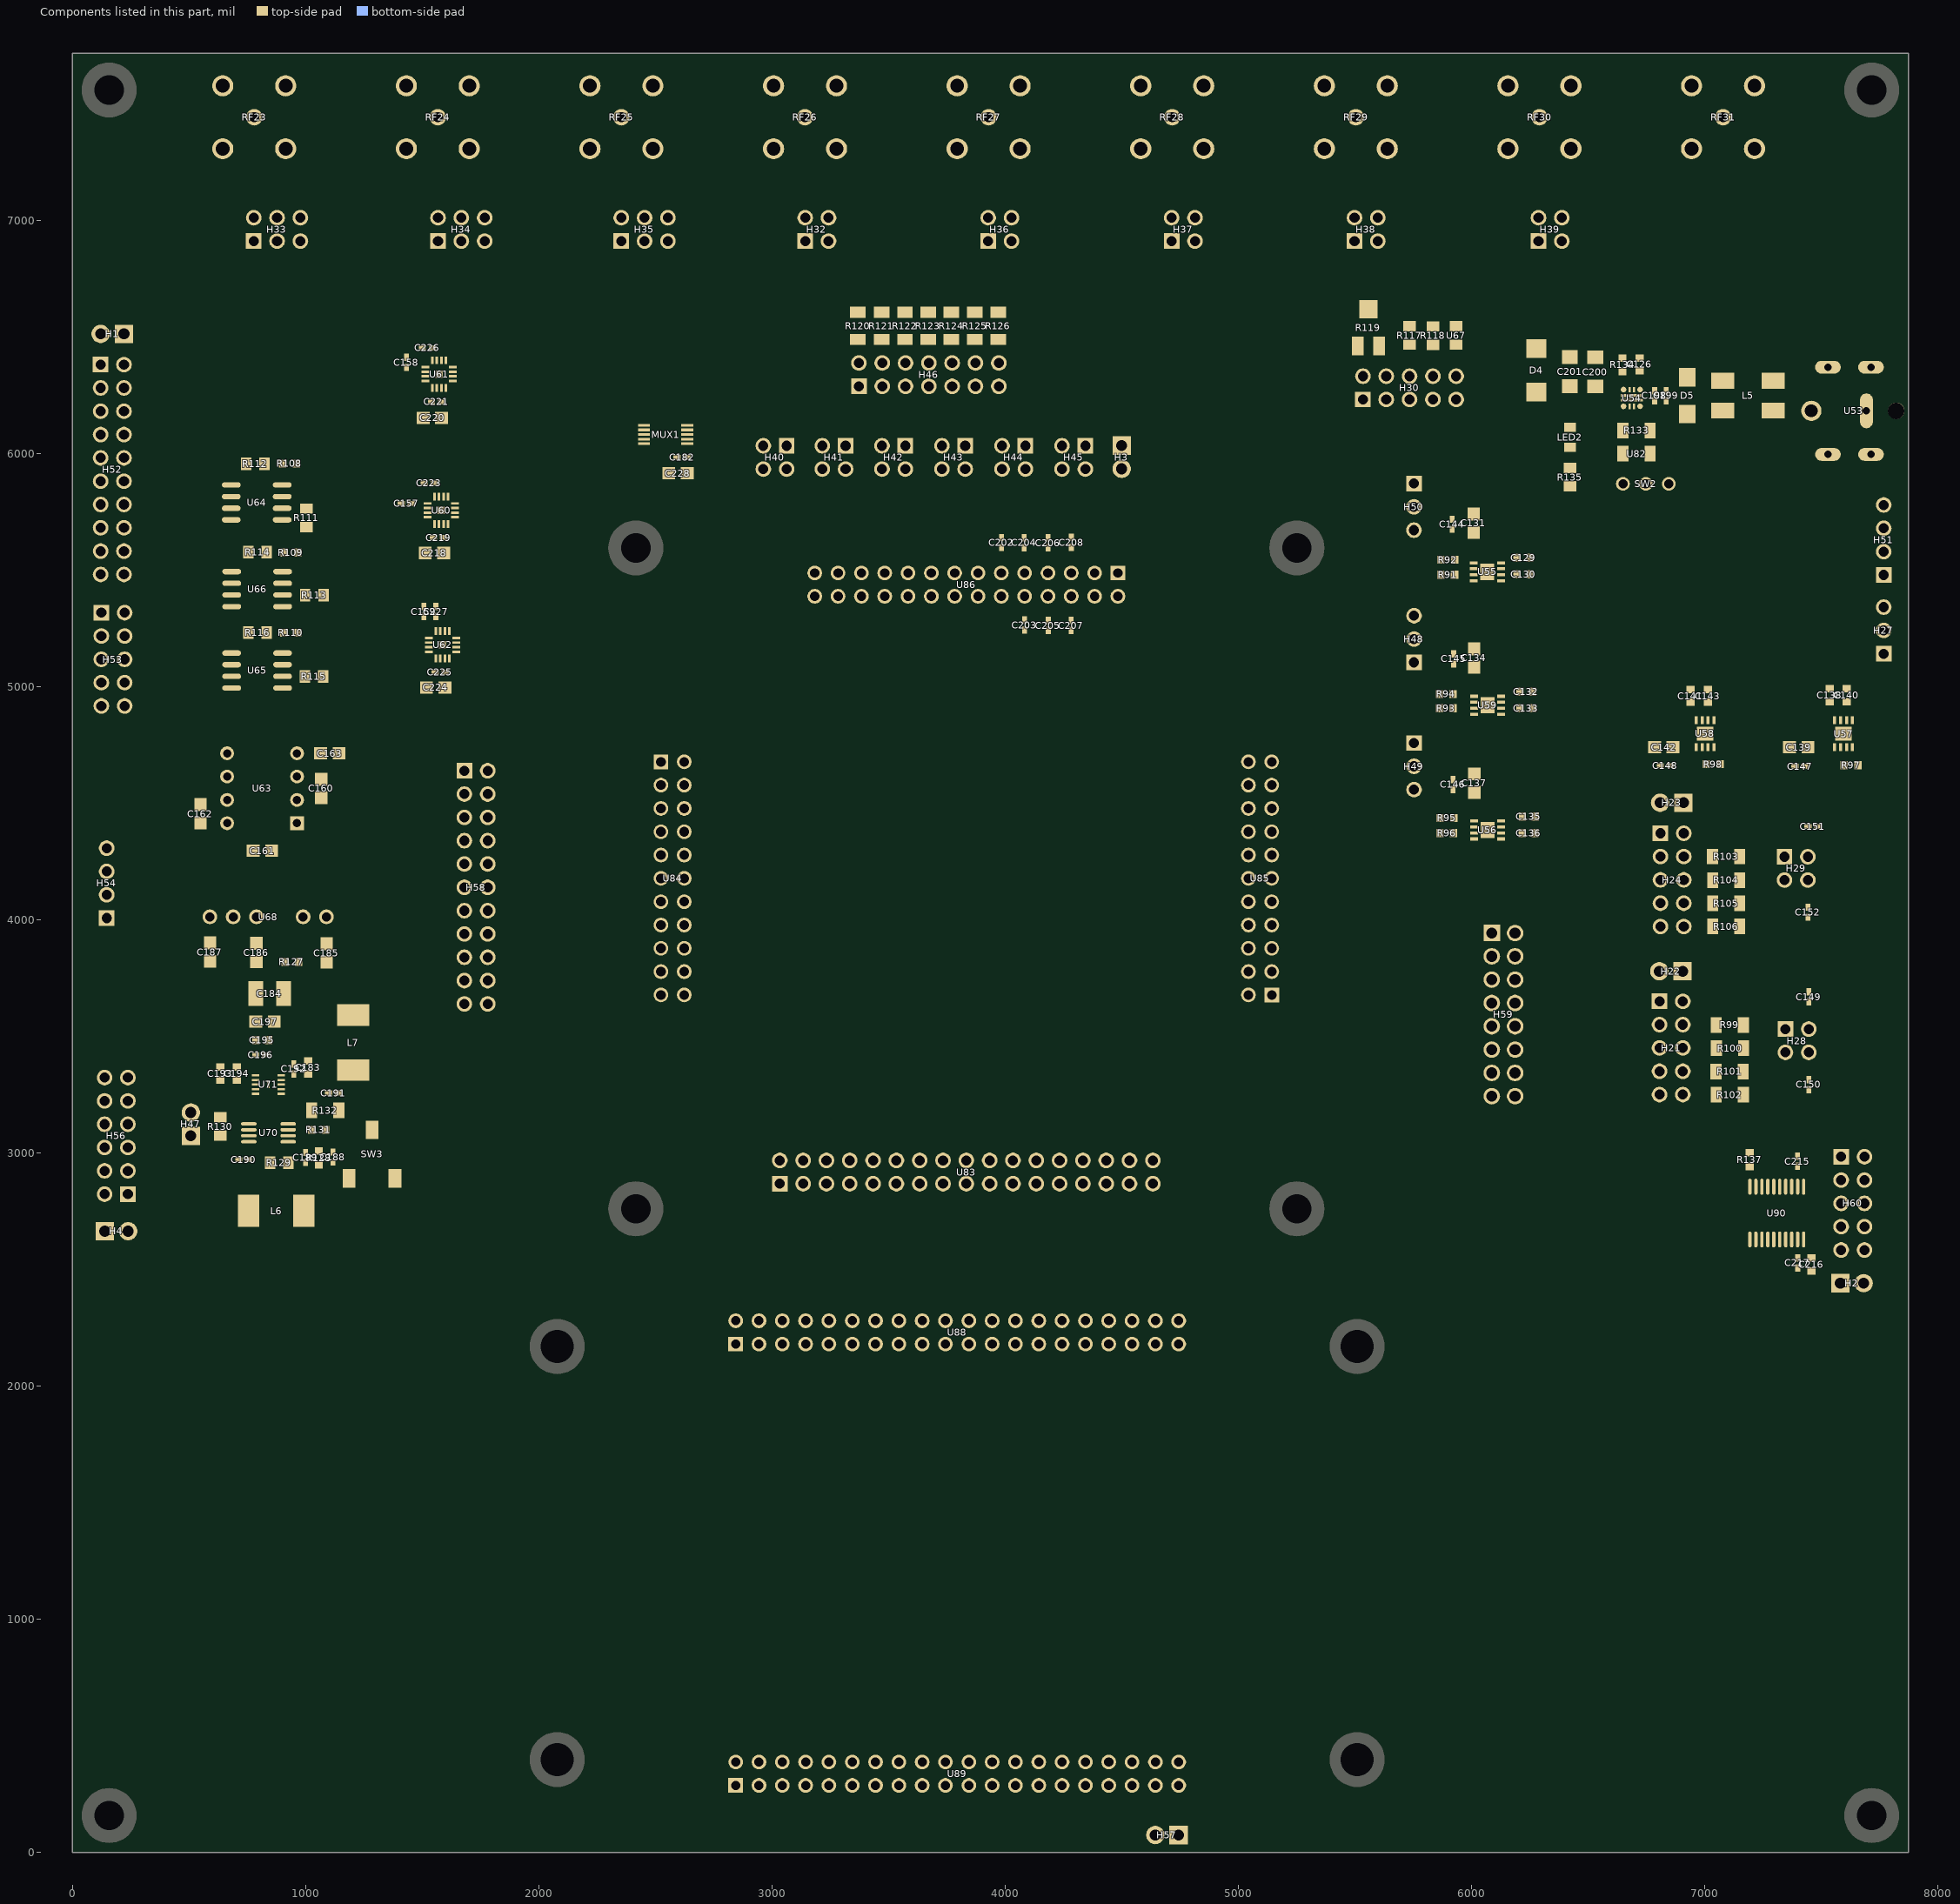
[diagram p0: the components of this part, seen from the top]
# Altium PCB MISC62793.pcbdoc (part 6 of 6)
Units mil, origin at the board's own origin, x right, y up, seen from the top; angles counter-clockwise.
Board outline 7874.02 x 7716.54 mil, 4 copper layers (Top Layer, GND, VCC, Bottom Layer); 201 components, 197 nets, 941 pads, 1215 vias.

## Polygon pours and split planes (outlines as drawn) (continued)
LDO_AVDD on Top Layer "Bottom Layer-No Net" (solid, remove dead copper, pour order 1005): 6837,4714 6837,4603 6847,4593 6869,4571 6917,4571 7325,4571 7371,4525 7410,4486 7410,4415 7410,4249 7421,4238 7422,4237 7442,4237 7481,4237 7485,4241 7492,4248 7492,4257 7492,4323 7472,4343 7460,4355 7460,4401 7460,4523 7387,4596 7358,4625 7238,4625 7047,4625 7032,4640 7022,4650 7022,4723 7022,4753 7020,4755 7019,4756 7014,4756 6923,4756 6916,4763 6910,4769 6898,4769 6847,4769 6840,4762 6837,4759 6837,4713
NetC198_2 on Top Layer "Bottom Layer-No Net" (solid, remove dead copper, pour order 1004): 6640,6231 6640,6226 6642,6224 6643,6223 6646,6223 6742,6223 6751,6214 6757,6208 6757,6199 6757,6164 6747,6154 6739,6146 6739,6133 6739,6072 6745,6066 6750,6061 6763,6061 7103,6061 7118,6076 7132,6090 7132,6150 7132,6209 7124,6217 7121,6220 7102,6220 6887,6220 6871,6236 6865,6242 6838,6242 6747,6242 6742,6237 6740,6235 6735,6235 6642,6235 6640,6233 6640,6230
5V on Top Layer "Bottom Layer-No Net" (solid, remove dead copper, pour order 1003): 175 vertices, not listed, extent 6109,4391 7823,6319
NetL5_1 on Top Layer "Bottom Layer-No Net" (solid, remove dead copper, pour order 1002): 7242,6160 7242,6110 7257,6095 7269,6083 7287,6083 7491,6083 7496,6088 7510,6102 7510,6139 7510,6208 7501,6217 7491,6227 7439,6227 7254,6227 7248,6221 7242,6215 7242,6162
TP_AVDD on Top Layer "Bottom Layer-No Net" (solid, remove dead copper, pour order 1001): 6871,4467 6871,4363 6890,4344 6897,4337 6910,4337 7081,4337 7103,4315 7119,4299 7119,4261 7119,3939 7133,3925 7140,3918 7160,3918 7348,3918 7351,3921 7375,3945 7375,4171 7375,4480 7354,4501 7306,4549 7001,4549 6888,4549 6882,4543 6871,4532 6871,4468
TP_DVDD on Top Layer "Bottom Layer-No Net" (solid, remove dead copper, pour order 1000): 6867,3763 6867,3740 6867,3637 6880,3624 6888,3616 6907,3616 7110,3616 7123,3603 7141,3585 7141,3329 7141,3219 7147,3213 7157,3203 7172,3203 7341,3203 7347,3209 7383,3245 7383,3455 7383,3764 7347,3800 7321,3826 7006,3826 6878,3826 6869,3817 6867,3815 6867,3762
0V on Top Layer "Bottom Layer-No Net" (solid, remove dead copper, pour order 1000): 450,3824 450,3806 450,3779 455,3774 478,3751 612,3751 907,3751 919,3763 926,3770 926,3794 926,3835 925,3836 914,3847 791,3847 458,3847 451,3840 450,3839 450,3825
VSS on Top Layer "Bottom Layer-No Net" (solid, remove dead copper, pour order 1001): -500,7458 -500,-256 -348,-408 -310,-446 296,-446 8238,-446 8352,-332 8485,-199 8485,-67 8485,7950 8276,8159 8086,8349 7442,8349 -36,8349 -301,8084 -490,7895 -490,7524
VSS on Bottom Layer "Bottom Layer-No Net" (solid, remove dead copper, pour order 1002): -635,7149 -635,49 -192,-394 68,-654 952,-654 8339,-654 8599,-394 8807,-186 8807,178 8807,8267 8339,8735 7845,9229 6336,9229 -271,9229 -687,8813 -609,8735 -609,7279
VSS on GND (split plane): 7853.92,20.1 20.1,20.1 20.1,2858.91 1143,2858.91 1145.61,2859.26 1148.04,2860.26 1150.13,2861.87 1270.13,2981.87 1271.74,2983.96 1272.74,2986.39 1273.09,2989 1273.09,3244 1272.74,3246.61 1271.74,3249.04 1270.13,3251.13 1221.13,3300.13 1219.04,3301.74 1216.61,3302.74 1214,3303.09 1096,3303.09 1093.39,3302.74 1092.17,3302.24 1090.96,3301.74 1088.87,3300.13 996.82,3208.09 658.18,3208.09 587.09,3279.18 587.09,3495.82 770.13,3678.87 771.74,3680.96 772.45,3682.68 772.74,3683.39 773.09,3686 773.09,4063 772.74,4065.61 771.74,4068.04 770.13,4070.13 709.13,4131.13 707.04,4132.74 704.61,4133.74 702,4134.09 20.1,4134.09 20.1,7696.44 7853.92,7696.44
0V on GND (split plane): 752.91,4058.82 752.91,3690.18 569.87,3507.13 568.27,3505.04 567.26,3502.61 566.91,3500 566.91,3275 567.26,3272.39 568.27,3269.96 569.87,3267.87 646.87,3190.87 648.96,3189.26 651.39,3188.26 654,3187.91 1001,3187.91 1003.61,3188.26 1006.04,3189.26 1008.13,3190.87 1100.18,3282.91 1209.82,3282.91 1252.91,3239.82 1252.91,2993.18 1138.82,2879.09 20.1,2879.09 20.1,4113.91 697.82,4113.91
VSS on VCC (split plane): 667.74,3634 526.87,3493.13 525.27,3491.04 524.26,3488.61 523.91,3486 523.91,3207 524.26,3204.39 525.27,3201.96 526.87,3199.87 700.87,3025.87 702.96,3024.26 703.67,3023.97 705.39,3023.26 708,3022.91 2180.91,3022.91 2180.91,2455 2181.26,2452.39 2182.27,2449.96 2183.87,2447.87 2595.87,2035.87 2597.96,2034.26 2598.67,2033.97 2600.39,2033.26 2603,2032.91 6120,2032.91 6122.61,2033.26 6125.04,2034.26 6127.13,2035.87 6610.18,2518.91 7167.82,2518.91 7289.87,2396.87 7291.96,2395.26 7293.17,2394.76 7294.39,2394.26 7297,2393.91 7853.92,2393.91 7853.92,20.1 20.1,20.1 20.1,3765.91 535.82,3765.91
DAC_VDD on VCC (split plane): 7853.92,5904.09 6424,5904.09 6421.39,5903.74 6418.96,5902.74 6416.87,5901.13 6134.82,5619.09 5708.18,5619.09 5519.13,5808.13 5517.04,5809.74 5514.61,5810.74 5512,5811.09 2377.18,5811.09 2242.09,5946.18 2242.09,6384 2241.74,6386.61 2240.74,6389.04 2239.13,6391.13 2054.13,6576.13 2052.04,6577.74 2049.61,6578.74 2047,6579.09 1566,6579.09 1563.39,6578.74 1561.67,6578.03 1560.96,6577.74 1558.87,6576.13 1486.87,6504.13 1485.27,6502.04 1484.26,6499.61 1483.91,6497 1483.91,6315 1484.26,6312.39 1485.27,6309.96 1486.87,6307.87 1534.87,6259.87 1536.96,6258.26 1539.39,6257.26 1542,6256.91 1704.82,6256.91 1771.91,6189.82 1771.91,6043.18 1729.82,6001.09 1530,6001.09 1527.39,6000.74 1524.96,5999.74 1522.87,5998.13 1443.87,5919.13 1442.27,5917.04 1441.26,5914.61 1440.91,5912 1440.91,5759 1441.26,5756.39 1442.27,5753.96 1443.87,5751.87 1502.87,5692.87 1504.96,5691.26 1507.39,5690.26 1510,5689.91 1715.82,5689.91 1757.91,5647.82 1757.91,5498.18 1707.82,5448.09 1537,5448.09 1534.39,5447.74 1533.68,5447.45 1531.96,5446.74 1529.87,5445.13 1459.87,5375.13 1458.27,5373.04 1457.26,5370.61 1456.91,5368 1456.91,5233 1457.26,5230.39 1458.27,5227.96 1459.87,5225.87 1516.87,5168.87 1518.96,5167.26 1519.67,5166.97 1521.39,5166.26 1524,5165.91 1613.82,5165.91 1664.91,5114.82 1664.91,5034.18 1288.87,4658.13 1287.27,4656.04 1286.26,4653.61 1285.91,4651 1285.91,3856.18 1073.82,3644.09 686.18,3644.09 547.13,3783.13 545.04,3784.74 542.61,3785.74 540,3786.09 20.1,3786.09 20.1,7696.44 7853.92,7696.44
3P3V on VCC (split plane): 2221.91,6379.82 2221.91,5942 2222.26,5939.39 2223.27,5936.96 2224.87,5934.87 2365.87,5793.87 2367.96,5792.26 2370.39,5791.26 2373,5790.91 5507.82,5790.91 5696.87,5601.87 5698.96,5600.26 5701.39,5599.26 5704,5598.91 6139,5598.91 6141.61,5599.26 6144.04,5600.26 6146.13,5601.87 6428.18,5883.91 7853.92,5883.91 7853.92,2414.09 7301.18,2414.09 7186.26,2529 7465.13,2807.87 7466.73,2809.96 7467.24,2811.17 7467.74,2812.39 7468.09,2815 7468.09,3150 7467.74,3152.61 7466.73,3155.04 7465.13,3157.13 7398.13,3224.13 7174.09,3448.18 7174.09,4560 7173.74,4562.61 7172.73,4565.04 7171.13,4567.13 6884.13,4854.13 6882.04,4855.74 6879.61,4856.74 6877,4857.09 2420,4857.09 2417.39,4856.74 2414.96,4855.74 2412.87,4854.13 2183.87,4625.13 2182.27,4623.04 2181.26,4620.61 2180.91,4618 2180.91,3043.09 712.18,3043.09 544.09,3211.18 544.09,3481.82 686.18,3623.91 1078,3623.91 1080.61,3624.26 1083.04,3625.26 1085.13,3626.87 1303.13,3844.87 1304.74,3846.96 1305.03,3847.67 1305.74,3849.39 1306.09,3852 1306.09,4646.82 1682.13,5022.87 1683.74,5024.96 1684.45,5026.68 1684.74,5027.39 1685.09,5030 1685.09,5119 1684.74,5121.61 1684.03,5123.33 1683.74,5124.04 1682.13,5126.13 1625.13,5183.13 1623.04,5184.74 1620.61,5185.74 1618,5186.09 1528.18,5186.09 1477.09,5237.18 1477.09,5363.82 1541.18,5427.91 1712,5427.91 1714.61,5428.26 1717.04,5429.26 1719.13,5430.87 1775.13,5486.87 1776.74,5488.96 1777.03,5489.67 1777.74,5491.39 1778.09,5494 1778.09,5652 1777.74,5654.61 1776.74,5657.04 1775.13,5659.13 1727.13,5707.13 1725.04,5708.74 1722.61,5709.74 1720,5710.09 1514.18,5710.09 1461.09,5763.18 1461.09,5907.82 1534.18,5980.91 1734,5980.91 1736.61,5981.26 1739.04,5982.26 1741.13,5983.87 1789.13,6031.87 1790.74,6033.96 1791.74,6036.39 1792.09,6039 1792.09,6194 1791.74,6196.61 1791.03,6198.33 1790.74,6199.04 1789.13,6201.13 1716.13,6274.13 1714.04,6275.74 1711.61,6276.74 1709,6277.09 1546.18,6277.09 1504.09,6319.18 1504.09,6492.82 1570.18,6558.91 2042.82,6558.91
DVDD on VCC (split plane): 6897.91,4121.82 6897.91,2793 6898.26,2790.39 6899.27,2787.96 6900.87,2785.87 7147.65,2539.09 6606,2539.09 6603.39,2538.74 6600.96,2537.74 6598.87,2536.13 6115.82,2053.09 2607.18,2053.09 2201.09,2459.18 2201.09,3030.81 2201.74,3032.39 2202.09,3035 2201.74,3037.61 2201.09,3039.19 2201.09,4342.91 2742.82,4342.91 2776.91,4308.82 2776.91,3964.18 2740.82,3928.09 2466,3928.09 2463.39,3927.74 2462.17,3927.24 2460.96,3926.74 2458.87,3925.13 2408.87,3875.13 2407.27,3873.04 2406.26,3870.61 2405.91,3868 2405.91,3384 2406.26,3381.39 2407.27,3378.96 2408.87,3376.87 2580.87,3204.87 2582.96,3203.26 2584.68,3202.55 2585.39,3202.26 2588,3201.91 3255.82,3201.91 3372.91,3084.82 3372.91,2826 3373.26,2823.39 3374.27,2820.96 3375.87,2818.87 3419.87,2774.87 3421.96,2773.26 3424.39,2772.26 3427,2771.91 3837,2771.91 3839.61,2772.26 3842.04,2773.26 3844.13,2774.87 3889.13,2819.87 3890.74,2821.96 3891.74,2824.39 3892.09,2827 3892.09,3033.82 4199.18,3340.91 5135,3340.91 5137.61,3341.26 5140.04,3342.26 5142.13,3343.87 5291.13,3492.87 5292.73,3494.96 5293.74,3497.39 5294.09,3500 5294.09,3662 5293.74,3664.61 5292.73,3667.04 5291.13,3669.13 5232.13,3728.13 5230.04,3729.74 5227.61,3730.74 5225,3731.09 5112.18,3731.09 5081.09,3762.18 5081.09,4019.82 5104.18,4042.91 5615,4042.91 5617.61,4043.26 5620.04,4044.26 5622.13,4045.87 5983.18,4406.91 6612.82,4406.91
1P8V on VCC (split plane): 7153.91,4555.82 7153.91,3444 7154.26,3441.39 7155.27,3438.96 7156.87,3436.87 7383.87,3209.87 7447.91,3145.82 7447.91,2819.18 7172,2543.26 6918.09,2797.18 6918.09,4126 6917.74,4128.61 6917.45,4129.32 6916.73,4131.04 6915.13,4133.13 6624.13,4424.13 6622.04,4425.74 6619.61,4426.74 6617,4427.09 5979,4427.09 5976.39,4426.74 5975.68,4426.45 5973.96,4425.74 5971.87,4424.13 5610.82,4063.09 5100,4063.09 5097.39,4062.74 5094.96,4061.74 5092.87,4060.13 5063.87,4031.13 5062.27,4029.04 5061.26,4026.61 5060.91,4024 5060.91,3758 5061.26,3755.39 5062.27,3752.96 5063.87,3750.87 5100.87,3713.87 5102.96,3712.26 5105.39,3711.26 5108,3710.91 5220.82,3710.91 5273.91,3657.82 5273.91,3504.18 5130.82,3361.09 4195,3361.09 4192.39,3360.74 4189.96,3359.74 4187.87,3358.13 3874.87,3045.13 3873.27,3043.04 3872.26,3040.61 3871.91,3038 3871.91,2831.18 3832.82,2792.09 3431.18,2792.09 3393.09,2830.18 3393.09,3089 3392.74,3091.61 3391.74,3094.04 3390.13,3096.13 3267.13,3219.13 3265.04,3220.74 3262.61,3221.74 3260,3222.09 2592.18,3222.09 2426.09,3388.18 2426.09,3863.82 2470.18,3907.91 2745,3907.91 2747.61,3908.26 2750.04,3909.26 2752.13,3910.87 2794.13,3952.87 2795.74,3954.96 2796.03,3955.67 2796.74,3957.39 2797.09,3960 2797.09,4313 2796.74,4315.61 2796.45,4316.32 2795.74,4318.04 2794.13,4320.13 2754.13,4360.13 2752.04,4361.74 2749.61,4362.74 2747,4363.09 2201.09,4363.09 2201.09,4613.82 2424.18,4836.91 6872.82,4836.91

## Keep-outs
Board Outline Layer:
  the board outline again, w5

## Other copper
GND (plane layer: these items are gaps in the copper):
  lines w20: 2,4124 702,4124 763,4063 763,3686 577,3500 577,3275 654,3198 1001,3198 1096,3293 1214,3293 1263,3244 1263,2989 1143,2869 12,2869
VCC (plane layer: these items are gaps in the copper):
  lines w20: 2,3776 540,3776 680,3636 680,3632 534,3486 534,3207 708,3033 2190,3033 2192,3035 ; 682,3634 1078,3634 1296,3852 1296,4651 1675,5030 1675,5119 1618,5176 1524,5176 1467,5233 1467,5368 1537,5438 1712,5438 1768,5494 1768,5652 1720,5700 1510,5700 1451,5759 1451,5912 1530,5991 1734,5991 1782,6039 1782,6194 1709,6267 1542,6267 1494,6315 1494,6497 1566,6569 2047,6569 2232,6384 2232,5942 2373,5801 5512,5801 5704,5609 6139,5609 6424,5894 7872,5894 ; 2197,4353 2747,4353 2787,4313 2787,3960 2745,3918 2466,3918 2416,3868 2416,3384 2588,3212 3260,3212 3383,3089 3383,2826 3427,2782 3837,2782 3882,2827 3882,3038 4195,3351 5135,3351 5284,3500 5284,3662 5225,3721 5108,3721 5071,3758 5071,4024 5100,4053 5615,4053 5979,4417 6617,4417 6908,4126 6908,2793 7297,2404 7876,2404 7874,2402 ; 2191,2455 2603,2043 6120,2043 6606,2529 7172,2529 7458,2815 7458,3150 7391,3217 7164,3444 7164,4560 6877,4847 5838,4847 2420,4847 2191,4618 2191,2455

## Silkscreen, mask and mechanical layers (free items; w line width, h text height)
Top Silkscreen Layer:
  lines w3.94: 2258.85,2602.66 2258.85,5752.27 5408.46,5752.27 5408.46,2602.66 2258.85,2602.66
  lines w5: 1901.88,220.46 5686.92,220.46 5686.92,2346.45 1901.88,2346.45 1901.88,220.46
  text "BNC6" at 4643,7162 h60
  text "BNC1" at 712,7161 h60
  text "BNC4" at 3069,7161 h60
  text "BNC5" at 3851,7161 h60
  text "VSS" at 7037,7161 h60
  text "BNC3" at 2284,7159 h60
  text "BNC8" at 6218,7157 h60
  text "BNC2" at 1496,7156 h60
  text "BNC7" at 5426,7155 h60
  text "VSS" at 291,6502 h40
  text "VSS" at 391,6501 h40
  text "VSL_TIA" at 291,6373 h40
  text "VSL_DAC" at 481,6372 h40
  text "DAC_REF2" at 484,6275 h40
  text "ADC_REF" at 289,6274 h40
  text "VB_CMP" at 302,6173 h40
  text "VTH_CMP" at 486,6170 h40
  text "DAC_REF1" at 484,6073 h40
  text "NCSVB" at 302,6069 h40
  text "VB_CLAMP" at 296,5968 h40
  text "VCLAMP" at 513,5966 h40
  text "VCB" at 477,5876 h40
  text "VB_CM" at 308,5874 h40
  text "VMH" at 517,5773 h40
  text "DAC_REF3" at 301,5772 h40
  text "5V" at 7642,5768 h40
  text "5V" at 7642,5681 h40
  text "TEST_VB" at 473,5677 h40
  text "VMH_DAC" at 280,5675 h40
  text "5V" at 7642,5581 h40
  text "VML" at 494,5568 h40
  text "VML_DAC" at 292,5567 h40
  text "N_5V" at 534,5473 h40
  text "NEG_5V_DAC" at 283,5471 h40
  text "EN_LDO" at 7554,5467 h40
  text "VSS" at 7619,5337 h40
  text "DAC3_OUT3" at 289,5311 h40
  text "NC" at 548,5306 h40
  text "VSS" at 7619,5232 h40
  text "DAC3_OUT5" at 284,5209 h40
  text "DAC3_OUT4" at 500,5207 h40
  text "VSS" at 7618,5132 h40
  text "D3_OUT7" at 288,5108 h40
  text "D3_OUT6" at 476,5107 h40
  text "SL_TEST" at 476,5008 h40
  text "WL_TEST" at 290,5006 h40
  text "BL_TEST" at 505,4907 h40
  text "TEST_OUT" at 292,4903 h40
  text "MODE" at 1853,4631 h40
  text "COL_ADDR7" at 1399,4622 h40
  text "COL_ADDR5" at 1397,4531 h40
  text "COL_ADDR6" at 1853,4530 h40
  text "COL_ADDR4" at 1856,4432 h40
  text "COL_ADDR3" at 1396,4430 h40
  text "COL_ADDR2" at 1853,4327 h40
  text "COL_ADDR1" at 1396,4324 h40
  text "OPA_NEG" at 211,4292 h40
  text "COL_ADDR0" at 1851,4228 h40
  text "COL_ADDR_EN" at 1346,4223 h40
  text "OPA_POS" at 214,4192 h40
  text "COL_CTRL" at 1853,4125 h40
  text "WE_CTRL" at 1431,4123 h40
  text "TIA_-5V" at 223,4092 h40
  text "WL_CTRL" at 1853,4030 h40
  text "WL_D_ADDR1" at 1367,4028 h40
  text "TIA_+5V" at 214,3996 h40
  text "ADC_TEST_EN" at 5746,3938 h40
  text "ADC_OUT7" at 6258,3932 h40
  text "WL_ADDR1" at 1407,3930 h40
  text "WL_D_ADDR0" at 1855,3929 h40
  text "ADC_OUT5" at 6257,3834 h40
  text "ADC_OUT6" at 5808,3833 h40
  text "WL_ADDR0" at 1851,3830 h40
  text "ROW_L_EN" at 1398,3827 h40
  text "ADC_OUT4" at 5811,3736 h40
  text "ADC_OUT3" at 6257,3733 h40
  text "RST_N" at 1449,3729 h40
  text "CLK" at 1857,3729 h40
  text "ADC_OUT2" at 5822,3631 h40
  text "ADC_OUT1" at 6257,3628 h40
  text "ROW_D_EN" at 1858,3627 h40
  text "DRIVER_TEST" at 1366,3618 h40
  text "ADC_OUT0" at 5815,3534 h40
  text "REG_STATE" at 6261,3533 h40
  text "REG_R_EN" at 5816,3430 h40
  text "REG_W_EN" at 6265,3427 h40
  text "CAL" at 5917,3337 h40
  text "ADC_EN" at 6256,3332 h40
  text "D_SDI" at 463,3322 h40
  text "D_SCLK" at 295,3320 h40
  text "ADC_RST" at 6256,3231 h40
  text "SAMPLE" at 5875,3227 h40
  text "CS2" at 298,3214 h40
  text "CS1" at 382,3212 h40
  text "SEL1" at 294,3111 h40
  text "CS3" at 386,3111 h40
  text "SEL0" at 295,3010 h40
  text "DIN" at 392,3007 h40
  text "NC" at 7762,2973 h40
  text "OUT0" at 7437,2970 h40
  text "ADC_SCLK" at 474,2911 h40
  text "SL_MUX" at 309,2910 h40
  text "OUT1" at 7760,2876 h40
  text "OUT2" at 7436,2873 h40
  text "ADC_OUT" at 494,2811 h40
  text "ADC_CNV" at 303,2808 h40
  text "OUT3" at 7763,2774 h40
  text "OUT4" at 7446,2772 h35
  text "R_3V3" at 7752,2677 h40
  text "E_3V3" at 7440,2676 h35
  text "VSS" at 313,2650 h40
  text "VSS" at 413,2649 h40
  text "M_3V3" at 7434,2589 h35
  text "T_3V3" at 7755,2578 h40
  text "VSS" at 7544,2346 h40
  text "VSS" at 7649,2344 h40
  text "COMPANY_A" at 7754,713 h120 r90